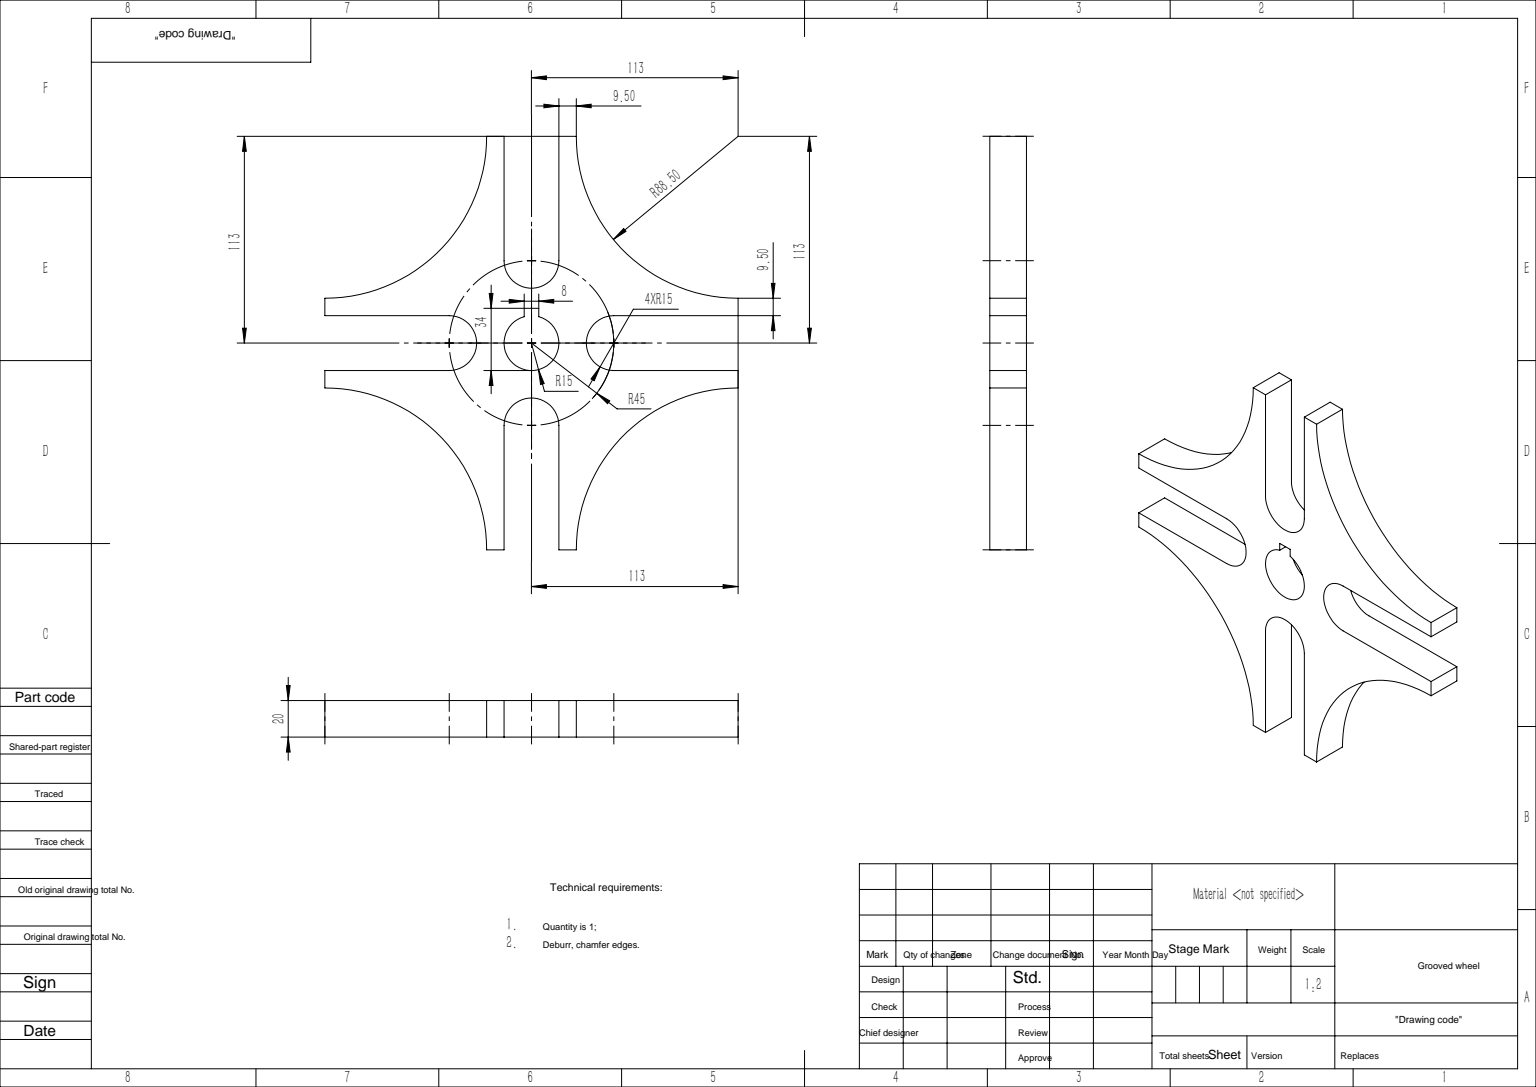
SolidWorks part; units mm, degrees
ref_plane "前视基准面" through (0, 0, 0) normal (0, 0, 1) x (1, 0, 0)
ref_plane "上视基准面" through (0, 0, 0) normal (0, 1, 0) x (1, 0, 0)
ref_plane "右视基准面" through (0, 0, 0) normal (1, 0, 0) x (0, 0, -1)
sketch "草图1" plane through (0, 0, 0) normal (0, 0, 1) x (1, 0, 0)
  line L0 (-150, 0) -> (150, 0) construction
  line L1 (0, 150) -> (0, -150) construction
  line L2 (45, 15) -> (113, 15)
  line L3 (15, -45) -> (15, -113)
  line L4 (24.5, -113) -> (15, -113)
  line L5 (113, -15) -> (45, -15)
  line L6 (113, 24.5) -> (113, 15)
  line L7 (15, 113) -> (15, 45)
  line L8 (113, -15) -> (113, -24.5)
  line L9 (15, 113) -> (24.5, 113)
  line L10 (-45, -15) -> (-113, -15)
  line L11 (-113, -24.5) -> (-113, -15)
  line L12 (-15, -113) -> (-15, -45)
  line L13 (-15, -113) -> (-24.5, -113)
  line L14 (-15, 45) -> (-15, 113)
  line L15 (-24.5, 113) -> (-15, 113)
  line L16 (-113, 15) -> (-45, 15)
  line L17 (-113, 15) -> (-113, 24.5)
  circle A0 centre (0, 0) radius 45 construction
  arc A1 (45, 15) -> (30, 0) centre (45, 0) ccw
  arc A2 (0, 30) -> (15, 45) centre (0, 45) ccw
  arc A3 (24.5, 113) -> (113, 24.5) centre (113, 113) ccw
  arc A4 (30, 0) -> (45, -15) centre (45, 0) ccw
  arc A5 (113, -24.5) -> (24.5, -113) centre (113, -113) ccw
  arc A6 (15, -45) -> (0, -30) centre (0, -45) ccw
  arc A7 (0, -30) -> (-15, -45) centre (0, -45) ccw
  arc A8 (-24.5, -113) -> (-113, -24.5) centre (-113, -113) ccw
  arc A9 (-45, -15) -> (-30, 0) centre (-45, 0) ccw
  arc A10 (-30, 0) -> (-45, 15) centre (-45, 0) ccw
  arc A11 (-113, 24.5) -> (-24.5, 113) centre (-113, 113) ccw
  arc A12 (-15, 45) -> (0, 30) centre (0, 45) ccw
  point P54 (0, 0)
  dimension "D1" = 90
  dimension "D4" = 30
  dimension "D5" = 177
  dimension "D2" = 300
  dimension "D3" = 300
  dimension "D6" = 113
  dimension "D7" = 113
  dimension "D8" = 113
  dimension "D9" = 113
  dimension "D10" = 4
extrude "凸台-拉伸1" add sketch "草图1" along normal blind 20
sketch "草图2" plane through (0, 0, 20) normal (0, 0, 1) x (1, 0, 0)
  line L0 (0, 0) -> (0, 40) construction
  line L1 (-4, 19) -> (4, 19)
  line L2 (-4, 19) -> (-4, 14.4568)
  line L4 (4, 19) -> (4, 14.4568)
  arc A0 (-4, 14.4568) -> (4, 14.4568) centre (0, 0) ccw
  dimension "D1" = 40
  dimension "D2" = 30
  dimension "D3" = 19
  dimension "D4" = 8
extrude "切除-拉伸1" cut sketch "草图2" against normal through all
